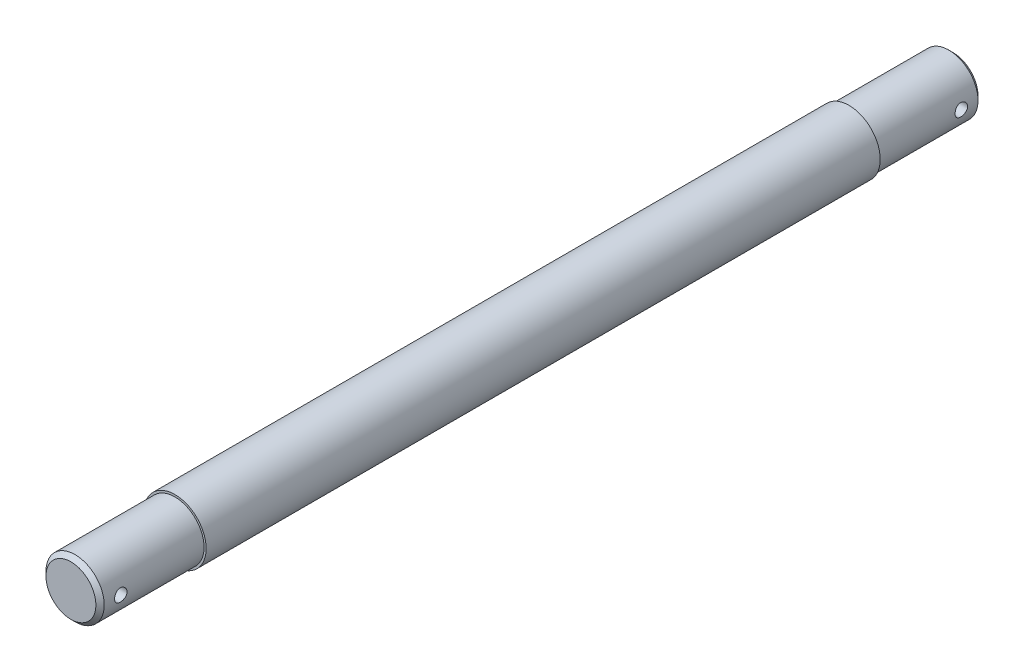
from build123d import *

# Parameters (mm, degrees)
SKETCH1_W               = 25
SKETCH1_H               = 7
CUT_EXTRUDE1_DEPTH      = 213.265164358
CUT_EXTRUDE1_DEPTH_BACK = 213.265164358
SKETCH2_R               = 1.5
CHAMFER1_SIZE           = 1


with BuildPart() as part:
    # Sketch1 → Revolve1 (revolve)
    with BuildSketch(Plane(origin=(0, 0, 0), x_dir=(0, 0, -1), z_dir=(1, 0, 0)), mode=Mode.PRIVATE) as revolve1_sk:
        with Locations((12.5, 3.5)):
            Rectangle(SKETCH1_W, SKETCH1_H)
        Polygon((25, 7), (25, 0), (187, 0), (187, 7), (187, 7.5), (25, 7.5), align=None)
        with Locations((199.5, 3.5)):
            Rectangle(SKETCH1_W, SKETCH1_H)
    revolve(revolve1_sk.sketch.rotate(Axis((0, 0, -25), (0, 0, -1)), 90), axis=Axis((0, 0, -25), (0, 0, -1)))

    # Sketch2 → Cut-Extrude1 (cut, two sides: drawn at the far end of the back side and taken through both)
    with BuildSketch(Plane(origin=(0, 0, 0), x_dir=(0, 0, -1), z_dir=(1, 0, 0)).offset(-CUT_EXTRUDE1_DEPTH_BACK)):
        with Locations((5, 0)):
            Circle(SKETCH2_R)
        with Locations((207, 0)):
            Circle(SKETCH2_R)
    extrude(amount=CUT_EXTRUDE1_DEPTH + CUT_EXTRUDE1_DEPTH_BACK, mode=Mode.SUBTRACT)

    # Chamfer1
    chamfer1_edges = [part.edges().sort_by_distance(p)[0] for p in [
        (-7, 0, 0),
        (-7, 0, -212),
    ]]
    chamfer(chamfer1_edges, length=CHAMFER1_SIZE)


solid = part.part
